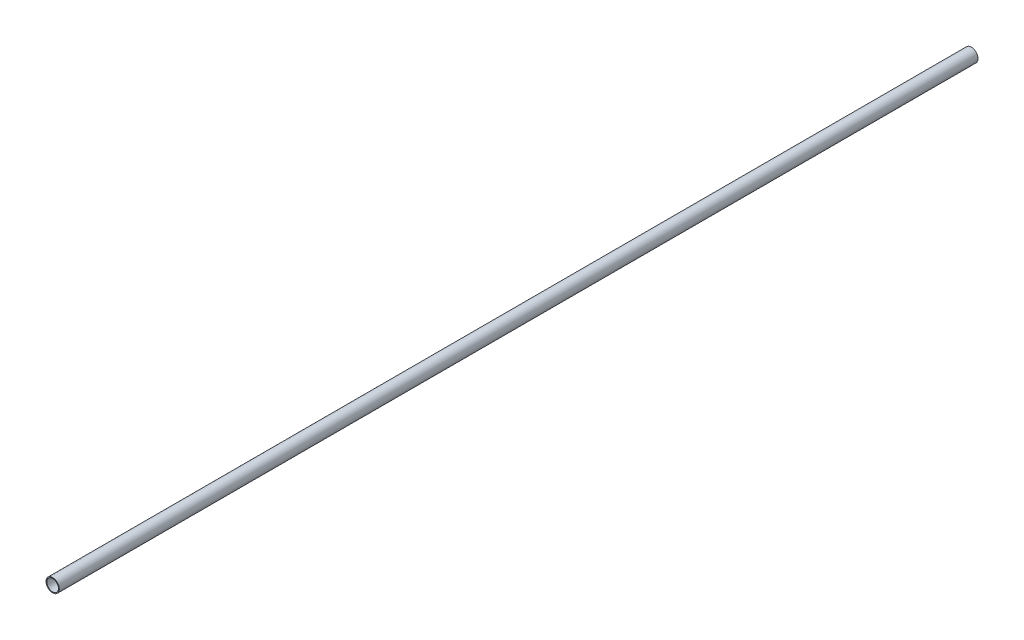
from build123d import *

# Parameters (mm, degrees)
SKETCH_1_R      = 16
SKETCH_1_R_2    = 14
EXTRUDE_1_DEPTH = 1105


with BuildPart() as part:
    # 草图1 → 凸台-拉伸1 (new, symmetric)
    with BuildSketch(Plane.XY):
        Circle(SKETCH_1_R)
        Circle(SKETCH_1_R_2, mode=Mode.SUBTRACT)
    extrude(amount=EXTRUDE_1_DEPTH, both=True)


solid = part.part
